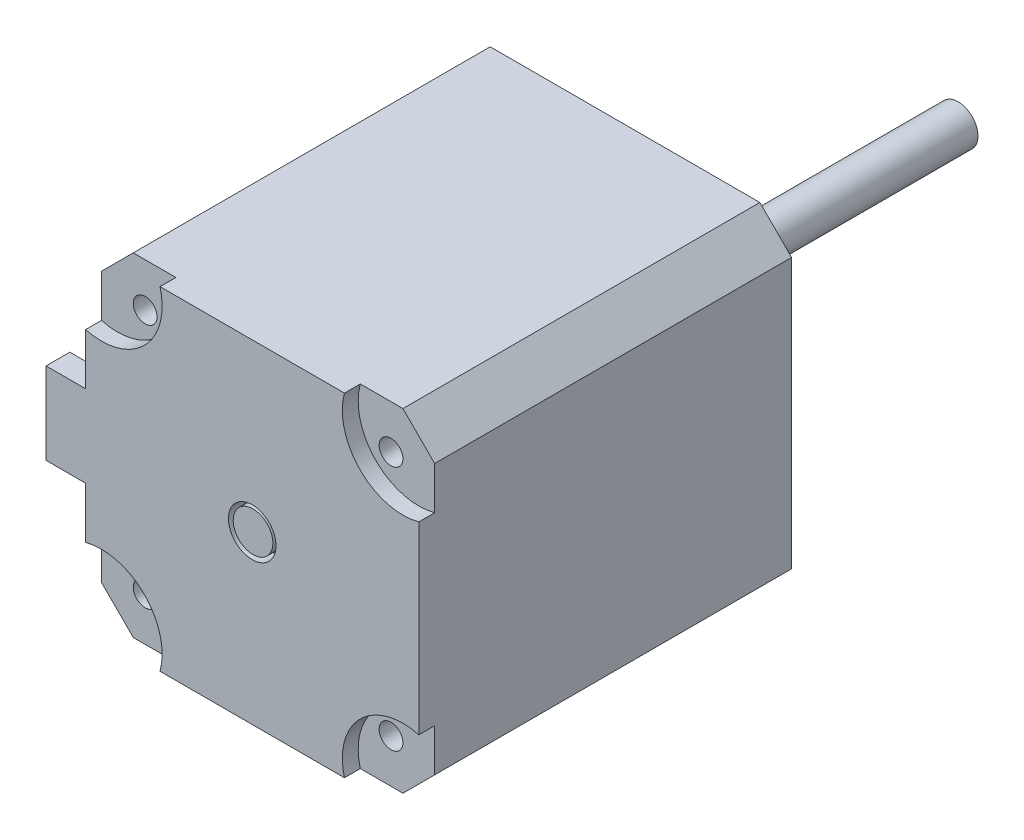
SolidWorks part; units mm, degrees
ref_plane "Front Plane" through (0, 0, 0) normal (0, 0, 1) x (1, 0, 0)
ref_plane "Top Plane" through (0, 0, 0) normal (0, 1, 0) x (1, 0, 0)
ref_plane "Right Plane" through (0, 0, 0) normal (1, 0, 0) x (0, 0, -1)
sketch "Sketch1" plane through (0, 0, 0) normal (0, 0, 1) x (1, 0, 0)
  line L0 (0, 21) -> (0, -21) construction
  line L1 (-21, 21) -> (21, 21)
  line L2 (-21, 21) -> (-21, -21)
  line L3 (-21, -21) -> (21, -21)
  line L4 (21, 21) -> (21, -21)
  line L5 (-21, 21) -> (21, -21) construction
  line L6 (-21, -21) -> (21, 21) construction
  line L7 (-21, 0) -> (21, 0) construction
  circle A0 centre (-15.5, 15.5) radius 1.5
  circle A1 centre (15.5, 15.5) radius 1.5
  circle A2 centre (-15.5, -15.5) radius 1.5
  circle A3 centre (15.5, -15.5) radius 1.5
  point P0 (0, 0)
  dimension "D2" = 31
  dimension "D3" = 3
  dimension "D1" = 42
  dimension "D4" = 42
extrude "Boss-Extrude1" add sketch "Sketch1" along normal blind 47
sketch "Sketch3" plane through (0, 0, 0) normal (0, 0, -1) x (-1, 0, 0)
  line L0 (-21, 17) -> (-17, 21)
  line L1 (-21, -21) -> (-21, 21) construction
  line L2 (-21, 21) -> (21, 21) construction
  line L3 (0, 18.9412) -> (0, -7.5636) construction
  line L4 (-16.264, 0) -> (-4.6279, 0) construction
  line L5 (-21, 21) -> (-21, 17)
  line L6 (-21, 21) -> (-17, 21)
  line L7 (21, 21) -> (17, 21)
  line L8 (21, 21) -> (21, 17)
  line L9 (21, 17) -> (17, 21)
  line L10 (21, -17) -> (17, -21)
  line L11 (21, -21) -> (21, -17)
  line L12 (21, -21) -> (17, -21)
  line L13 (-21, -21) -> (-17, -21)
  line L14 (-21, -21) -> (-21, -17)
  line L15 (-21, -17) -> (-17, -21)
  dimension "D1" = 4
  dimension "D2" = 4
extrude "Cut-Extrude1" cut sketch "Sketch3" against normal through all
sketch "Sketch4" plane through (0, 0, 0) normal (0, 0, -1) x (-1, 0, 0)
  circle A0 centre (0, 0) radius 11
  dimension "D1" = 22
extrude "Boss-Extrude2" add sketch "Sketch4" along normal blind 2
sketch "Sketch5" plane through (0, 0, -2) normal (0, 0, -1) x (-1, 0, 0)
  line L0 (1.7, -1.833) -> (1.7, 1.833)
  arc A0 (1.7, 1.833) -> (1.7, -1.833) centre (0, 0) ccw
  dimension "D1" = 5
  dimension "D2" = 1.7
extrude "Boss-Extrude3" add sketch "Sketch5" along normal blind 40
sketch "Sketch7" plane through (0, 0, 47) normal (0, 0, 1) x (1, 0, 0)
  line L0 (-17, 21) -> (-21, 17) construction
  line L9 (0, 13.3214) -> (0, 5.5116) construction
  line L10 (-12.44, 0) -> (-6.0632, 0) construction
  line L11 (21, 17) -> (21, 11.6255)
  line L12 (17, 21) -> (21, 17)
  line L13 (11.6255, 21) -> (17, 21)
  line L14 (-21, -17) -> (-21, -11.6255)
  line L15 (-17, -21) -> (-21, -17)
  line L16 (-11.6255, -21) -> (-17, -21)
  line L17 (17, -21) -> (21, -17)
  line L18 (21, -17) -> (21, 17)
  line L19 (21, 17) -> (17, 21)
  line L20 (17, 21) -> (-17, 21)
  line L21 (-17, 21) -> (-21, 17)
  line L22 (-21, 17) -> (-21, -17)
  line L23 (-21, -17) -> (-17, -21)
  line L24 (-17, -21) -> (17, -21)
  line L28 (-11.6255, 21) -> (-17, 21)
  line L29 (-17, 21) -> (-21, 17)
  line L30 (-21, 17) -> (-21, 11.6255)
  line L33 (11.6255, -21) -> (17, -21)
  line L34 (17, -21) -> (21, -17)
  line L35 (21, -17) -> (21, -11.6255)
  arc A0 (-21, 11.6255) -> (-11.6255, 21) centre (-19, 19) ccw
  arc A1 (21, 11.6255) -> (11.6255, 21) centre (19, 19) cw
  arc A2 (21, -11.6255) -> (11.6255, -21) centre (19, -19) ccw
  arc A3 (-21, -11.6255) -> (-11.6255, -21) centre (-19, -19) cw
  dimension "D1" = 0
extrude "Cut-Extrude2" cut sketch "Sketch7" against normal blind 2
sketch "Sketch8" plane through (0, 0, 47) normal (0, 0, 1) x (1, 0, 0)
  circle A0 centre (0, 0) radius 3
  dimension "D1" = 6
extrude "Cut-Extrude3" cut sketch "Sketch8" against normal blind 2
sketch "Sketch9" plane through (0, 0, 45) normal (0, 0, 1) x (1, 0, 0)
  circle A0 centre (0, 0) radius 2.5
  dimension "D1" = 5
extrude "Boss-Extrude4" add sketch "Sketch9" along normal blind 1.9
sketch "Sketch10" plane through (-21, 0, 0) normal (-1, 0, 0) x (0, 0, 1)
  line L5 (47, 11.6255) -> (47, -11.6255) construction
  line L6 (44, 5.155) -> (47, 5.155)
  line L7 (44, 5.155) -> (44, -5.155)
  line L8 (44, -5.155) -> (47, -5.155)
  line L9 (47, 5.155) -> (47, -5.155)
  line L10 (44, 5.155) -> (47, -5.155) construction
  line L11 (44, -5.155) -> (47, 5.155) construction
  line L13 (44.2607, 4.2591) -> (46.7393, 4.2591)
  line L14 (44.2607, 4.2591) -> (44.2607, -4.2591)
  line L15 (44.2607, -4.2591) -> (46.7393, -4.2591)
  line L16 (46.7393, 4.2591) -> (46.7393, -4.2591)
  line L17 (44.2607, 4.2591) -> (46.7393, -4.2591) construction
  line L18 (44.2607, -4.2591) -> (46.7393, 4.2591) construction
  point P0 (45.5, 0)
  point P7 (45.5, 0)
  dimension "D1" = 3
extrude "Boss-Extrude5" add sketch "Sketch10" along normal blind 5
sketch "Sketch11" plane through (-21, 0, 0) normal (-1, 0, 0) x (0, 0, 1)
  line L0 (45.5, 4.2591) -> (45.5, -4.2591) construction
  line L1 (46.7393, 4.2591) -> (44.2607, 4.2591) construction
  line L2 (44.2607, -4.2591) -> (46.7393, -4.2591) construction
  circle A0 centre (45.5, 3.1278) radius 0.5
  circle A1 centre (45.5, 1.6278) radius 0.5
  circle A2 centre (45.5, 0.1278) radius 0.5
  circle A3 centre (45.5, -1.3722) radius 0.5
  circle A4 centre (45.5, -2.8722) radius 0.5
  dimension "D1" = 1
  dimension "D2" = 5
extrude "Boss-Extrude6" add sketch "Sketch11" along normal blind 5
